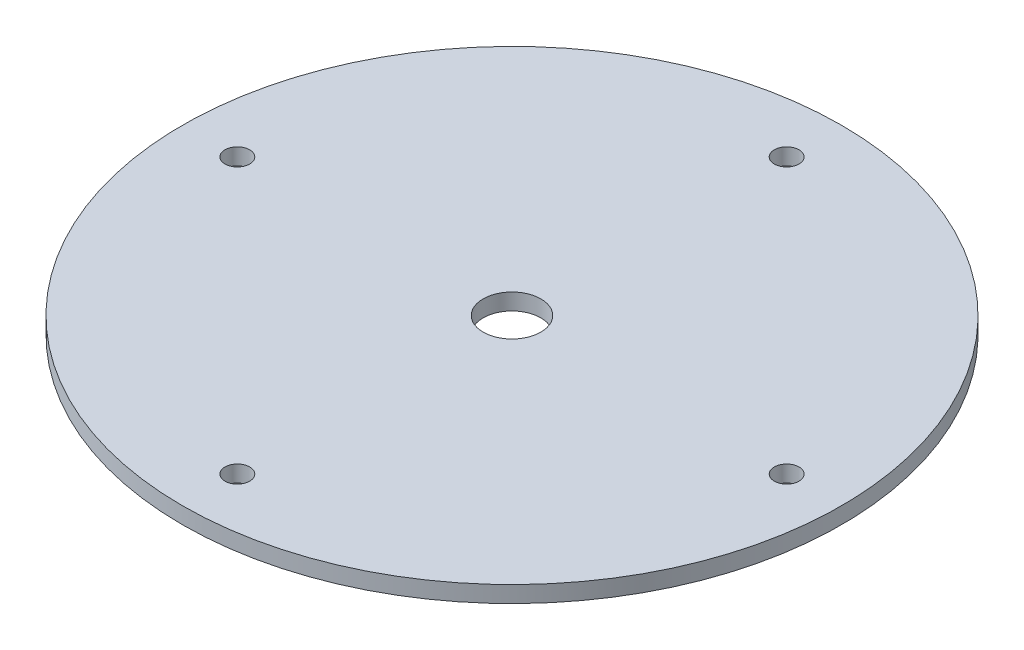
SolidWorks part; units mm, degrees
ref_plane "Front Plane" through (0, 0, 0) normal (0, 0, 1) x (1, 0, 0)
ref_plane "Top Plane" through (0, 0, 0) normal (0, 1, 0) x (1, 0, 0)
ref_plane "Right Plane" through (0, 0, 0) normal (1, 0, 0) x (0, 0, -1)
sketch "Sketch1" plane through (0, 0, 0) normal (0, 1, 0) x (1, 0, 0)
  circle A0 centre (0, 0) radius 40
  dimension "D1" = 80
extrude "Boss-Extrude1" add sketch "Sketch1" along normal blind 2
sketch "Sketch2" plane through (0, 0, 0) normal (0, -1, 0) x (1, 0, 0)
  circle A0 centre (0, 0) radius 3.5
extrude "Cut-Extrude3" cut sketch "Sketch2" against normal blind 52
sketch "Sketch3" plane through (0, 2, 0) normal (0, 1, 0) x (1, 0, 0)
  circle A0 centre (0, 0) radius 33.3387 construction
  circle A1 centre (0, 33.3387) radius 1.5
  circle A2 centre (33.3387, 0) radius 1.5
  circle A3 centre (0, -33.3387) radius 1.5
  circle A4 centre (-33.3387, 0) radius 1.5
  point P14 (0, 0)
  dimension "D1" = 3
  dimension "D2" = 4
extrude "Cut-Extrude4" cut sketch "Sketch3" against normal blind 45
